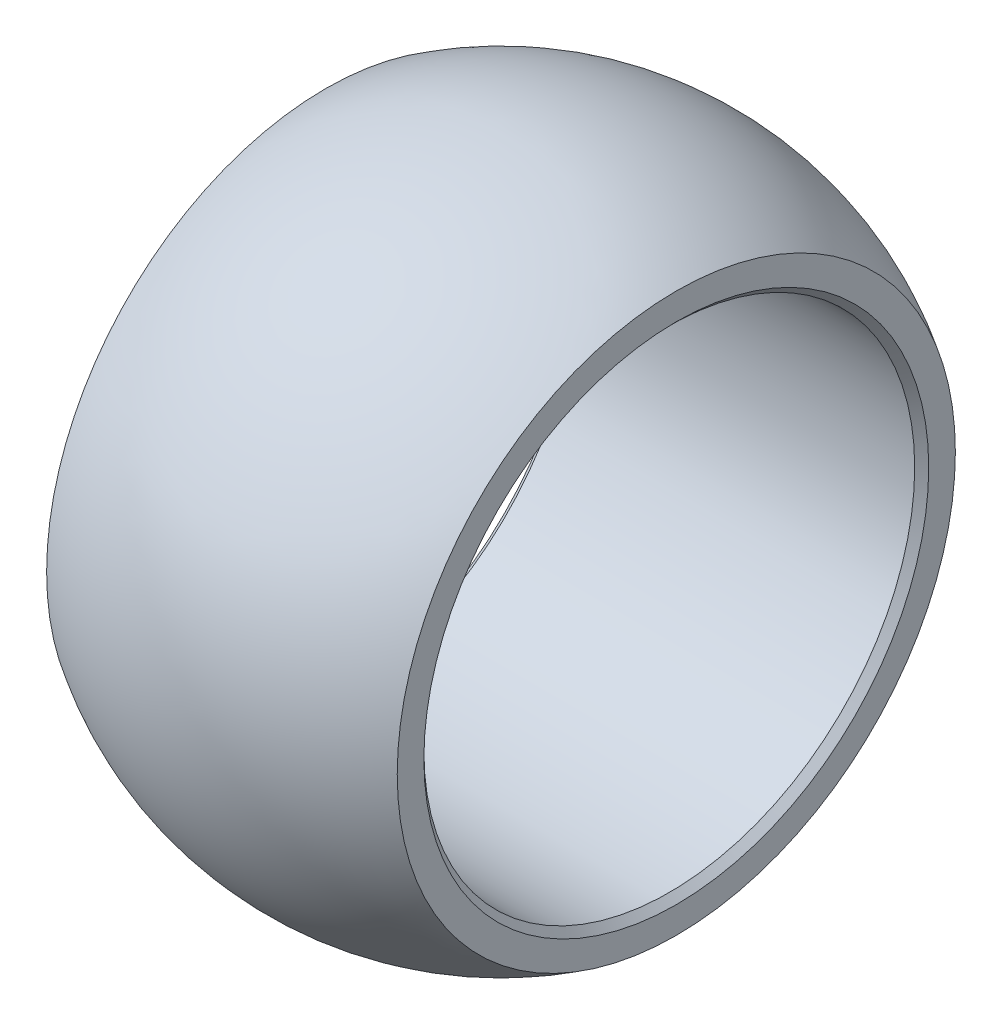
from build123d import *

# Parameters (mm, degrees)
CHAMFER_1_SIZE = 0.5


with BuildPart() as part:
    # 草图1 → 旋转1 (revolve)
    with BuildSketch(Plane.XY):
        with BuildLine():
            Line((-12.5, 19.899748742), (-12.5, 17.5))
            Line((-12.5, 17.5), (12.5, 17.5))
            Line((12.5, 17.5), (12.5, 19.899748742))
            ThreePointArc((12.5, 19.899748742), (0, 23.5), (-12.5, 19.899748742))
        make_face()
    revolve(axis=Axis((-75.39340763, 0, 0), (1, 0, 0)))

    # 倒角1
    chamfer_1_edges = [part.edges().sort_by_distance(p)[0] for p in [
        (12.5, -17.5, 0),
        (-12.5, -17.5, 0),
    ]]
    chamfer(chamfer_1_edges, length=CHAMFER_1_SIZE)


solid = part.part
